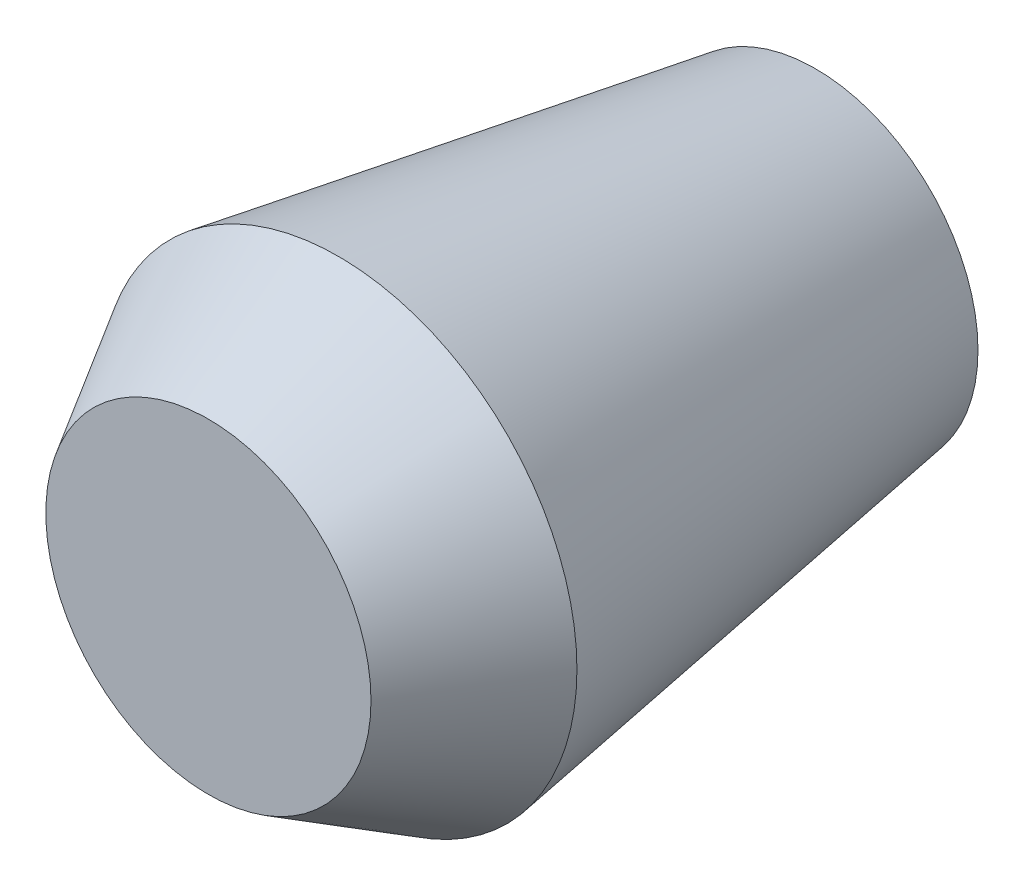
from build123d import *

# Parameters (mm, degrees)
M6_TAPPED_HOLE1_D     = 5
M6_TAPPED_HOLE1_DEPTH = 20
M6_TAPPED_HOLE1_TIP   = 1.502151548


with BuildPart() as part:
    # Sketch1 → Revolve1 (revolve)
    with BuildSketch(Plane(origin=(0, 0, 0), x_dir=(1, 0, 0), z_dir=(0, 1, 0)), mode=Mode.PRIVATE) as revolve1_sk:
        Polygon((0, 0), (-7.5, 0), (-11, 6), (-7.5, 28), (0, 28), align=None)
    revolve(revolve1_sk.sketch.rotate(Axis((0, 0, 0), (0, 0, -1)), 180), axis=Axis((0, 0, 0), (0, 0, -1)))

    # M6 Tapped Hole1
    with Locations(Plane(origin=(0, 0, -28), x_dir=(-1, 0, 0), z_dir=(0, 0, -1))):
        with Locations((0, 0)):
            Hole(M6_TAPPED_HOLE1_D / 2, depth=M6_TAPPED_HOLE1_DEPTH)
            with Locations((0, 0, -(M6_TAPPED_HOLE1_DEPTH + M6_TAPPED_HOLE1_TIP / 2))):  # 118° drill point
                Cone(0, M6_TAPPED_HOLE1_D / 2, M6_TAPPED_HOLE1_TIP, mode=Mode.SUBTRACT)


solid = part.part
